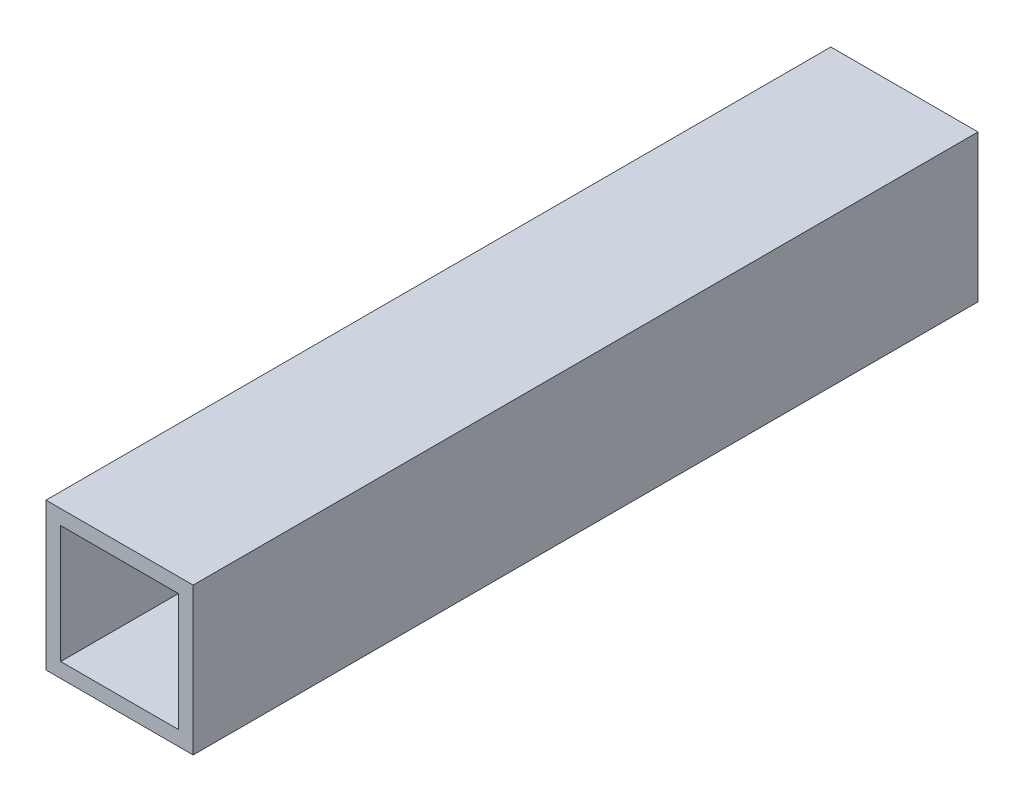
from build123d import *

# Parameters (mm, degrees)
SKETCH_1_W      = 30
SKETCH_1_H      = 30
SKETCH_1_W_2    = 24
SKETCH_1_H_2    = 24
EXTRUDE_1_DEPTH = 80


with BuildPart() as part:
    # 草图1 → 凸台-拉伸1 (new, symmetric)
    with BuildSketch(Plane.XY):
        Rectangle(SKETCH_1_W, SKETCH_1_H)
        Rectangle(SKETCH_1_W_2, SKETCH_1_H_2, mode=Mode.SUBTRACT)
    extrude(amount=EXTRUDE_1_DEPTH, both=True)


solid = part.part
